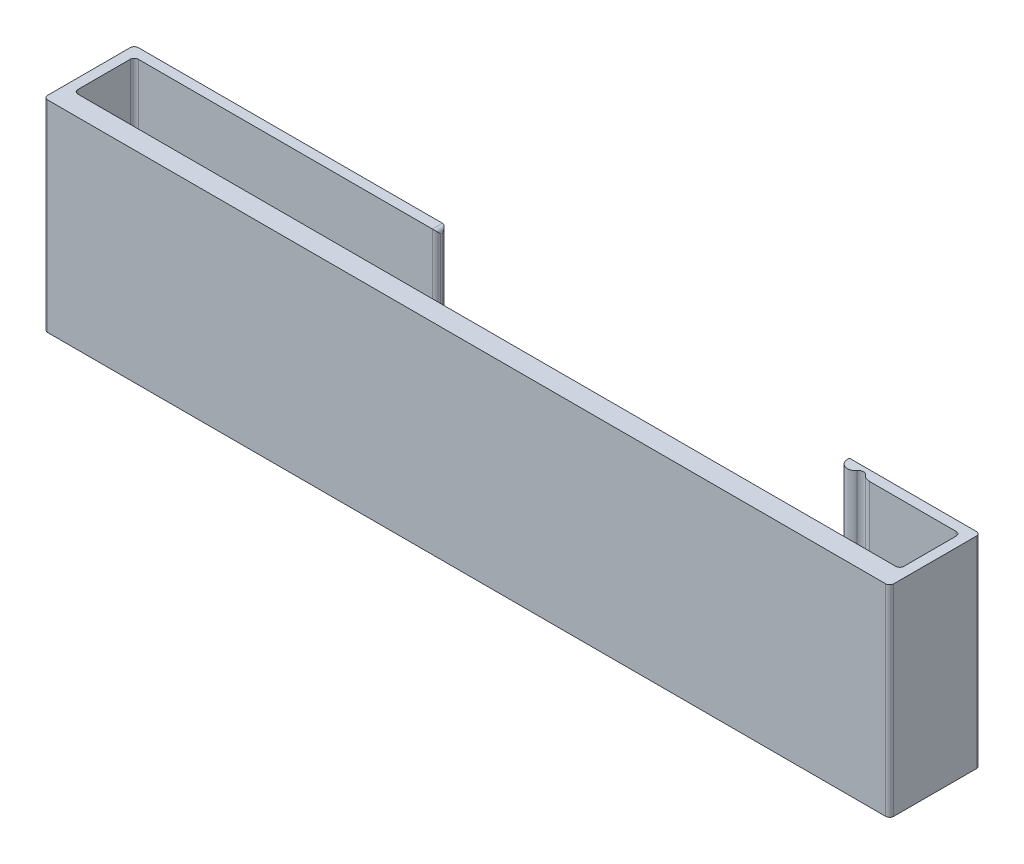
from build123d import *

# Parameters (mm, degrees)
SKETCH1_W           = 15.5
SKETCH1_H           = 10
BOSS_EXTRUDE1_DEPTH = 0.5
SKETCH2_W           = 0.5
SKETCH2_H           = 10
BOSS_EXTRUDE2_DEPTH = 3
SKETCH3_W           = 42
SKETCH3_H           = 10
BOSS_EXTRUDE3_DEPTH = 1
SKETCH4_W           = 0.5
SKETCH4_H           = 10
BOSS_EXTRUDE4_DEPTH = 4.5
BOSS_EXTRUDE5_DEPTH = 10
FILLET1_R           = 0.2


with BuildPart() as part:
    # Sketch1 → Boss-Extrude1 (new body)
    with BuildSketch(Plane.XY):
        with Locations((-134.781169153, 115.619026916)):
            Rectangle(SKETCH1_W, SKETCH1_H)
    extrude(amount=BOSS_EXTRUDE1_DEPTH)

    # Sketch2 → Boss-Extrude2 (add)
    with BuildSketch(Plane.XY.offset(0.5)):
        with Locations((-142.281169153, 115.619026916)):
            Rectangle(SKETCH2_W, SKETCH2_H)
    extrude(amount=BOSS_EXTRUDE2_DEPTH)

    # Sketch3 → Boss-Extrude3 (add)
    with BuildSketch(Plane.XY.offset(3.5)):
        with Locations((-121.531169153, 115.619026916)):
            Rectangle(SKETCH3_W, SKETCH3_H)
    extrude(amount=BOSS_EXTRUDE3_DEPTH)

    # Sketch4 → Boss-Extrude4 (add)
    with BuildSketch(Plane.XY.offset(4.5)):
        with Locations((-100.781169153, 115.619026916)):
            Rectangle(SKETCH4_W, SKETCH4_H)
    extrude(amount=-BOSS_EXTRUDE4_DEPTH)

    # Sketch6 → Boss-Extrude5 (add)
    with BuildSketch(Plane(origin=(0, 110.619026916, 0), x_dir=(-1, 0, 0), z_dir=(0, -1, 0))):
        with BuildLine():
            Line((100.531169153, 0), (107.031169153, 0))
            Line((107.031169153, 0), (107.031169153, -0.1))
            ThreePointArc((107.031169153, -0.1), (106.754872908, -0.48039109), (106.307682248, -0.335279031))
            ThreePointArc((106.307682248, -0.335279031), (106.114215823, -0.2324803), (105.914058339, -0.321552283))
            ThreePointArc((105.914058339, -0.321552283), (105.742384515, -0.453197607), (105.531169153, -0.5))
            Line((105.531169153, -0.5), (100.531169153, -0.5))
            Line((100.531169153, -0.5), (100.531169153, 0))
        make_face()
    extrude(amount=-BOSS_EXTRUDE5_DEPTH)

    # Fillet1
    fillet1_edges = [part.edges().sort_by_distance(p)[0] for p in [
        (-127.031169153, 115.619026916, 0.5),
        (-142.031169153, 115.619026916, 0.5),
        (-142.031169153, 115.619026916, 3.5),
        (-142.531169153, 115.619026916, 4.5),
        (-100.531169153, 115.619026916, 4.5),
        (-100.531169153, 115.619026916, 0),
        (-101.031169153, 115.619026916, 3.5),
        (-127.031169153, 115.619026916, 0),
        (-142.531169153, 115.619026916, 0),
        (-101.031169153, 115.619026916, 0.5),
        (-127.031169153, 120.619026916, 0.25),
        (-127.031169153, 110.619026916, 0.25),
    ]]
    fillet(fillet1_edges, radius=FILLET1_R)


solid = part.part
